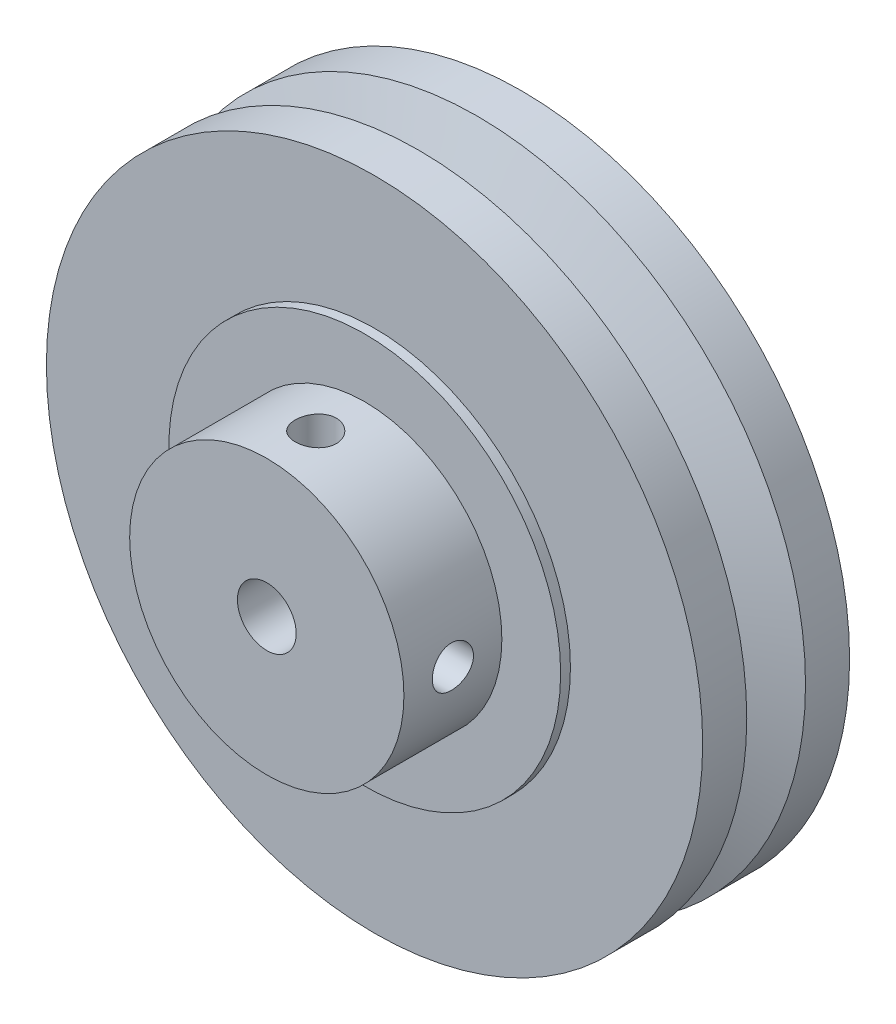
from build123d import *

# Parameters (mm, degrees)
SKETCH1_R                       = 33.5
BOSS_EXTRUDE1_DEPTH             = 15
SKETCH4_R                       = 14
BOSS_EXTRUDE2_DEPTH             = 11
SKETCH3_R                       = 20
BOSS_EXTRUDE4_DEPTH             = 2
BOSS_EXTRUDE3_START             = 1
SKETCH2_R                       = 20
BOSS_EXTRUDE3_DEPTH             = 1
SKETCH5_R                       = 3
CUT_EXTRUDE3_DEPTH              = 56.031808984
M5_TAPPED_HOLE1_D               = 4.2
M5_TAPPED_HOLE1_DEPTH           = 13
M5_TAPPED_HOLE1_TIP             = 1.2618073
M5_TAPPED_HOLE1_ON_FACE_2_D     = 4.2
M5_TAPPED_HOLE1_ON_FACE_2_DEPTH = 13
M5_TAPPED_HOLE1_ON_FACE_2_TIP   = 1.2618073


with BuildPart() as part:
    # Sketch1 → Boss-Extrude1 (new body)
    with BuildSketch(Plane.XY):
        Circle(SKETCH1_R)
    extrude(amount=BOSS_EXTRUDE1_DEPTH)

    # Sketch4 → Boss-Extrude2 (add)
    with BuildSketch(Plane.XY.offset(15)):
        Circle(SKETCH4_R)
    extrude(amount=BOSS_EXTRUDE2_DEPTH)

    # Sketch3 → Boss-Extrude4 (add)
    with BuildSketch(Plane(origin=(0, 0, 0), x_dir=(-1, 0, 0), z_dir=(0, 0, -1))):
        Circle(SKETCH3_R)
    extrude(amount=BOSS_EXTRUDE4_DEPTH)

    # Sketch2 → Boss-Extrude3 (add)
    with BuildSketch(Plane.XY.offset(15).offset(BOSS_EXTRUDE3_START)):
        with Locations(Location((0, 0, 0), (0, 0, 180))):
            Circle(SKETCH2_R)
    extrude(amount=-BOSS_EXTRUDE3_DEPTH)

    # Sketch5 → Cut-Extrude3 (cut, through all)
    with BuildSketch(Plane.XY.offset(26)):
        Circle(SKETCH5_R)
    extrude(amount=-CUT_EXTRUDE3_DEPTH, mode=Mode.SUBTRACT)

    # Sketch7 → Cut-Revolve1 (revolve, cut)
    with BuildSketch(Plane(origin=(0, 0, 0), x_dir=(0, 0, -1), z_dir=(1, 0, 0)), mode=Mode.PRIVATE) as cut_revolve1_sk:
        Polygon((-8, 26.85), (-7, 26.85), (-4.5, 33.5), (-10.5, 33.5), align=None)
    revolve(cut_revolve1_sk.sketch.rotate(Axis((0, 0, 0), (0, 0, 1)), 90), axis=Axis((0, 0, 0), (0, 0, 1)), mode=Mode.SUBTRACT)

    # M5 Tapped Hole1
    with Locations(Plane(origin=(0, 14, 21), x_dir=(1, 0, 0), z_dir=(0, 1, 0))):
        with Locations((0, 0)):
            Hole(M5_TAPPED_HOLE1_D / 2, depth=M5_TAPPED_HOLE1_DEPTH)
            with Locations((0, 0, -(M5_TAPPED_HOLE1_DEPTH + M5_TAPPED_HOLE1_TIP / 2))):  # 118° drill point
                Cone(0, M5_TAPPED_HOLE1_D / 2, M5_TAPPED_HOLE1_TIP, mode=Mode.SUBTRACT)

    # M5 Tapped Hole1 on face 2
    with Locations(Plane(origin=(14, 0, 21), x_dir=(0, 0, 1), z_dir=(1, 0, 0))):
        with Locations((0, 0)):
            Hole(M5_TAPPED_HOLE1_ON_FACE_2_D / 2, depth=M5_TAPPED_HOLE1_ON_FACE_2_DEPTH)
            with Locations((0, 0, -(M5_TAPPED_HOLE1_ON_FACE_2_DEPTH + M5_TAPPED_HOLE1_ON_FACE_2_TIP / 2))):  # 118° drill point
                Cone(0, M5_TAPPED_HOLE1_ON_FACE_2_D / 2, M5_TAPPED_HOLE1_ON_FACE_2_TIP, mode=Mode.SUBTRACT)


solid = part.part
